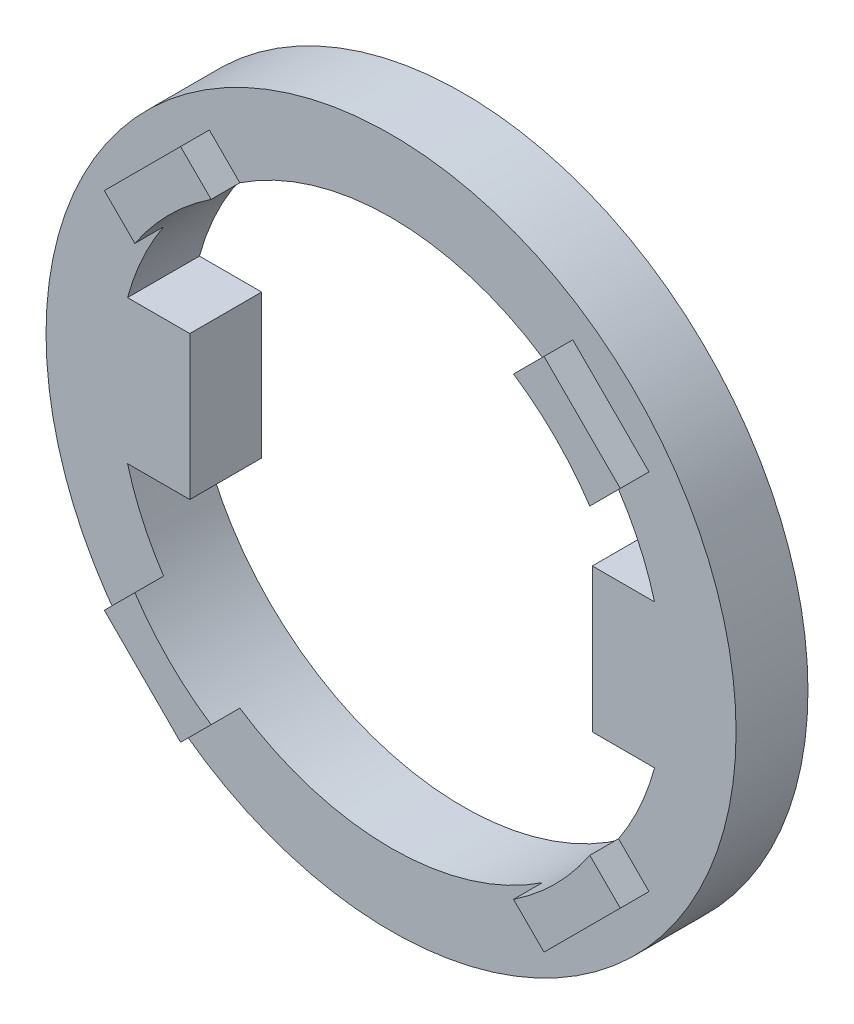
SolidWorks part; units mm, degrees
ref_plane "前视基准面" through (0, 0, 0) normal (0, 0, 1) x (1, 0, 0)
ref_plane "上视基准面" through (0, 0, 0) normal (0, 1, 0) x (1, 0, 0)
ref_plane "右视基准面" through (0, 0, 0) normal (1, 0, 0) x (0, 0, -1)
sketch "草图1" plane through (0, 0, 0) normal (0, 0, 1) x (1, 0, 0)
  line L0 (-19, 0) -> (19, 0) construction
  line L1 (-18.3303, 5) -> (-14, 5)
  line L2 (0, 19) -> (0, -19) construction
  line L3 (-18.3303, -5) -> (-14, -5)
  line L4 (-14, 5) -> (-14, -5)
  line L5 (18.3303, 5) -> (14, 5)
  line L6 (14, 5) -> (14, -5)
  line L7 (18.3303, -5) -> (14, -5)
  circle A0 centre (0, 0) radius 24
  arc A1 (-18.3303, -5) -> (18.3303, -5) centre (0, 0) ccw
  arc A2 (18.3303, 5) -> (-18.3303, 5) centre (0, 0) ccw
  dimension "D1" = 48
  dimension "D2" = 38
  dimension "D3" = 5
  dimension "D4" = 14
extrude "凸台-拉伸1" add sketch "草图1" along normal blind 5
sketch "草图2" plane through (0, 0, 5) normal (0, 0, 1) x (1, 0, 0)
  line L0 (0, 0) -> (0, 24) construction
  line L1 (0, 0) -> (-24, 0) construction
  line L2 (0, 0) -> (-18.3264, 18.3264) construction
  line L3 (-15.8224, 10.5191) -> (-17.9437, 12.6404)
  line L4 (-10.5191, 15.8224) -> (-12.6404, 17.9437)
  line L5 (-17.9437, 12.6404) -> (-12.6404, 17.9437)
  line L6 (10.5191, 15.8224) -> (12.6404, 17.9437)
  line L7 (12.6404, 17.9437) -> (17.9437, 12.6404)
  line L8 (15.8224, 10.5191) -> (17.9437, 12.6404)
  line L9 (15.8224, -10.5191) -> (17.9437, -12.6404)
  line L10 (17.9437, -12.6404) -> (12.6404, -17.9437)
  line L11 (10.5191, -15.8224) -> (12.6404, -17.9437)
  line L12 (-10.5191, -15.8224) -> (-12.6404, -17.9437)
  line L13 (-12.6404, -17.9437) -> (-17.9437, -12.6404)
  line L14 (-15.8224, -10.5191) -> (-17.9437, -12.6404)
  circle A0 centre (0, 0) radius 24 construction
  circle A1 centre (0, 0) radius 24 construction
  arc A2 (18.3303, 5) -> (-18.3303, 5) centre (0, 0) ccw construction
  arc A3 (15.8224, 10.5191) -> (10.5191, 15.8224) centre (0, 0) ccw
  arc A4 (-18.3303, -5) -> (18.3303, -5) centre (0, 0) ccw construction
  arc A5 (-15.8224, -10.5191) -> (-10.5191, -15.8224) centre (0, 0) ccw
  arc A6 (-10.5191, 15.8224) -> (-15.8224, 10.5191) centre (0, 0) ccw
  arc A7 (10.5191, -15.8224) -> (15.8224, -10.5191) centre (0, 0) ccw
  dimension "D1" = 45
  dimension "D2" = 7.5
  dimension "D3" = 3
  dimension "D4" = 4
extrude "凸台-拉伸2" add sketch "草图2" along normal blind 2
